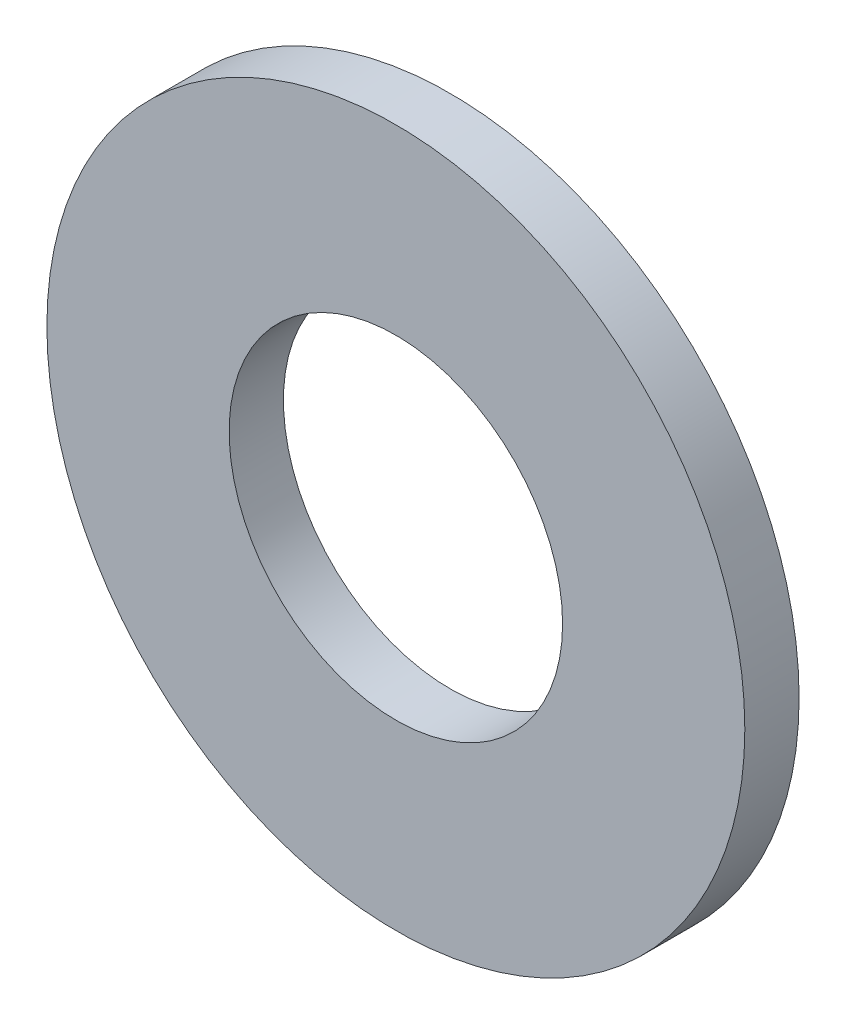
from build123d import *

# Parameters (mm, degrees)
SKETCH1_R           = 4.5
SKETCH1_R_2         = 2.15
BOSS_EXTRUDE1_DEPTH = 0.7


with BuildPart() as part:
    # Sketch1 → Boss-Extrude1 (new body)
    with BuildSketch(Plane.XY):
        Circle(SKETCH1_R)
        Circle(SKETCH1_R_2, mode=Mode.SUBTRACT)
    extrude(amount=BOSS_EXTRUDE1_DEPTH)


solid = part.part
